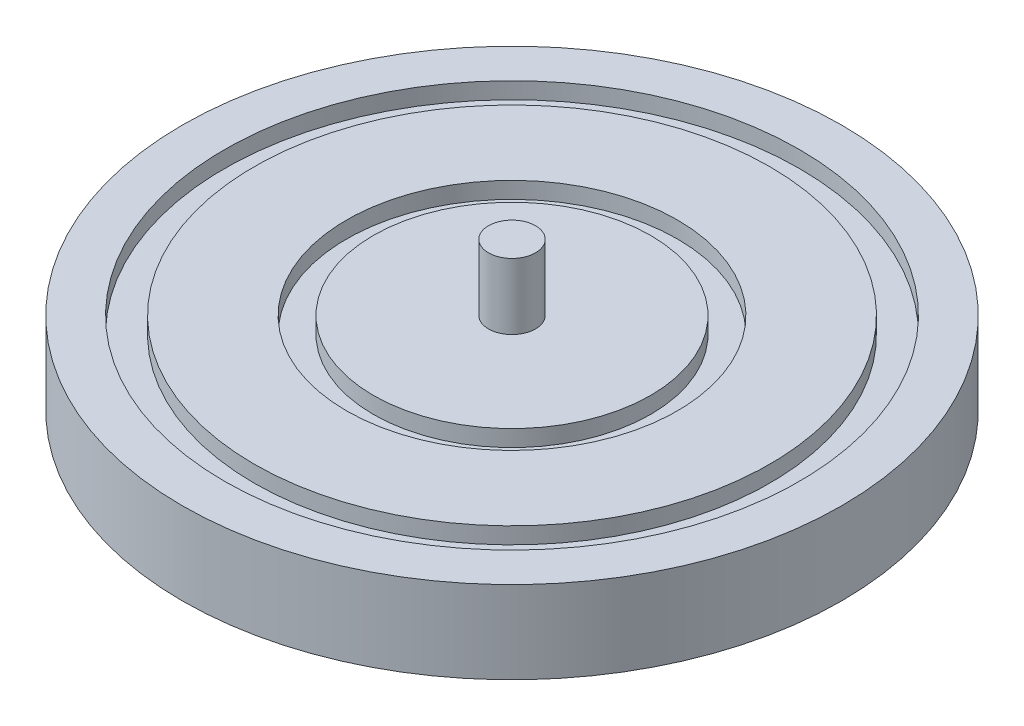
SolidWorks part; units mm, degrees
ref_plane "前视基准面" through (0, 0, 0) normal (0, 0, 1) x (1, 0, 0)
ref_plane "上视基准面" through (0, 0, 0) normal (0, 1, 0) x (1, 0, 0)
ref_plane "右视基准面" through (0, 0, 0) normal (1, 0, 0) x (0, 0, -1)
sketch "草图1" plane through (0, 0, 0) normal (0, 1, 0) x (1, 0, 0)
  circle A0 centre (0, 0) radius 20
  dimension "D1" = 40
extrude "凸台-拉伸1" add sketch "草图1" along normal blind 5
sketch "草图2" plane through (0, 0, 0) normal (0, -1, 0) x (1, 0, 0)
  circle A0 centre (0, 0) radius 5
  dimension "D1" = 10
extrude "凸台-拉伸2" add sketch "草图2" along normal blind 6
sketch "草图3" plane through (0, 0, 0) normal (0, -1, 0) x (1, 0, 0)
  circle A0 centre (0, 0) radius 9.5454
  circle A1 centre (0, 0) radius 11.6695
extrude "切除-拉伸1" cut sketch "草图3" against normal blind 1
sketch "草图4" plane through (0, 5, 0) normal (0, 1, 0) x (1, 0, 0)
  circle A0 centre (0, 0) radius 1.425
  dimension "D1" = 2.85
extrude "凸台-拉伸3" add sketch "草图4" along normal blind 4
sketch "草图5" plane through (0, 5, 0) normal (0, 1, 0) x (1, 0, 0)
  circle A0 centre (0, 0) radius 17.4353
  circle A1 centre (0, 0) radius 15.6342
extrude "切除-拉伸2" cut sketch "草图5" against normal blind 1
sketch "草图6" plane through (0, 5, 0) normal (0, 1, 0) x (1, 0, 0)
  circle A0 centre (0, 0) radius 10.0341
  circle A1 centre (0, 0) radius 8.4089
extrude "切除-拉伸3" cut sketch "草图6" against normal blind 1
